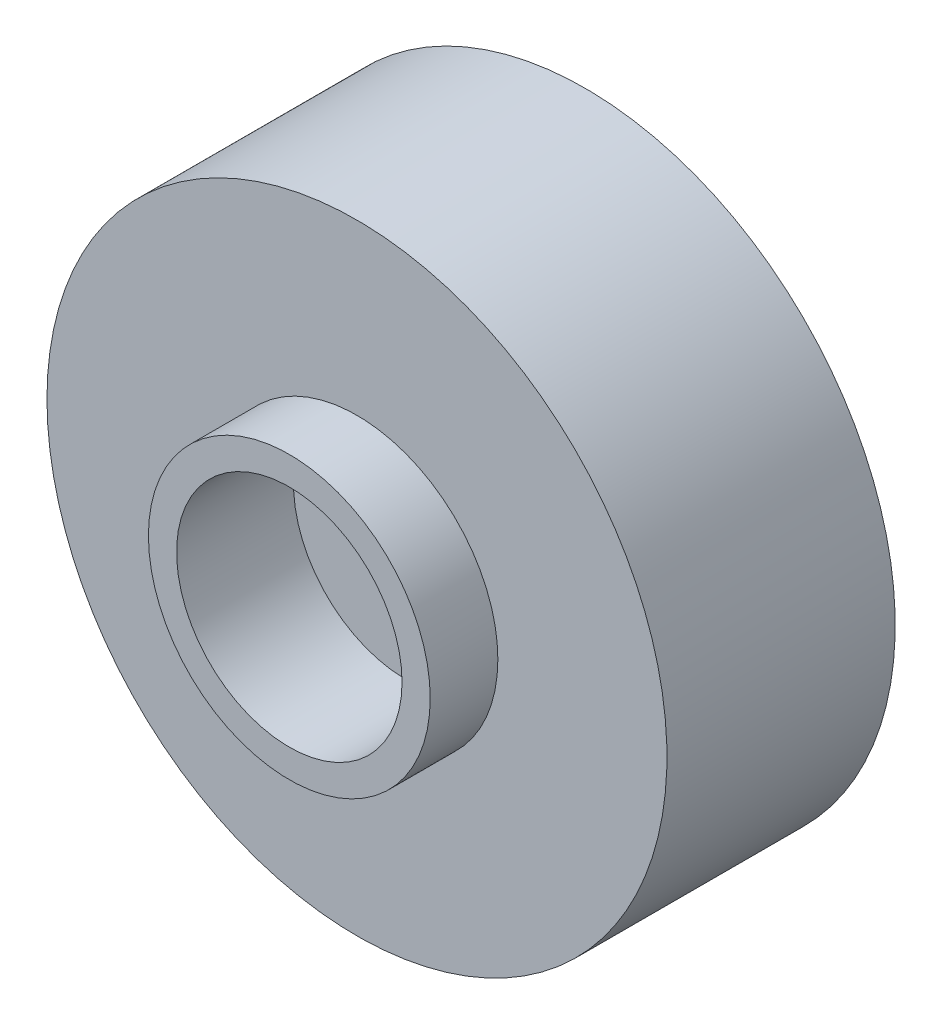
SolidWorks part; units mm, degrees
material "PEEK"
ref_plane "Front Plane" through (0, 0, 0) normal (0, 0, 1) x (1, 0, 0)
ref_plane "Top Plane" through (0, 0, 0) normal (0, 1, 0) x (1, 0, 0)
ref_plane "Right Plane" through (0, 0, 0) normal (1, 0, 0) x (0, 0, -1)
sketch "Sketch1" plane through (0, 0, 0) normal (0, 0, 1) x (1, 0, 0)
  circle A0 centre (0, 0) radius 11
  dimension "D1" = 22
extrude "Boss-Extrude1" add sketch "Sketch1" along normal blind 10.5
sketch "Sketch2" plane through (0, 0, 10.5) normal (0, 0, 1) x (1, 0, 0)
  circle A0 centre (0, 0) radius 5
  dimension "D1" = 10
extrude "Cut-Extrude1" cut sketch "Sketch2" against normal blind 2.4 flip side to cut
sketch "Sketch3" plane through (0, 0, 10.5) normal (0, 0, 1) x (1, 0, 0)
  circle A0 centre (0, 0) radius 4
  dimension "D1" = 8
extrude "Cut-Extrude2" cut sketch "Sketch3" against normal blind 4.15
sketch "Sketch4" plane through (0, 0, 0) normal (0, 0, -1) x (-1, 0, 0)
  circle A0 centre (0, 0) radius 8.75
  dimension "D1" = 17.5
extrude "Cut-Extrude3" cut sketch "Sketch4" against normal blind 3
chamfer "Chamfer1" distance 0.2 angle 45 1 edges at (-8.75, 0, 0)
